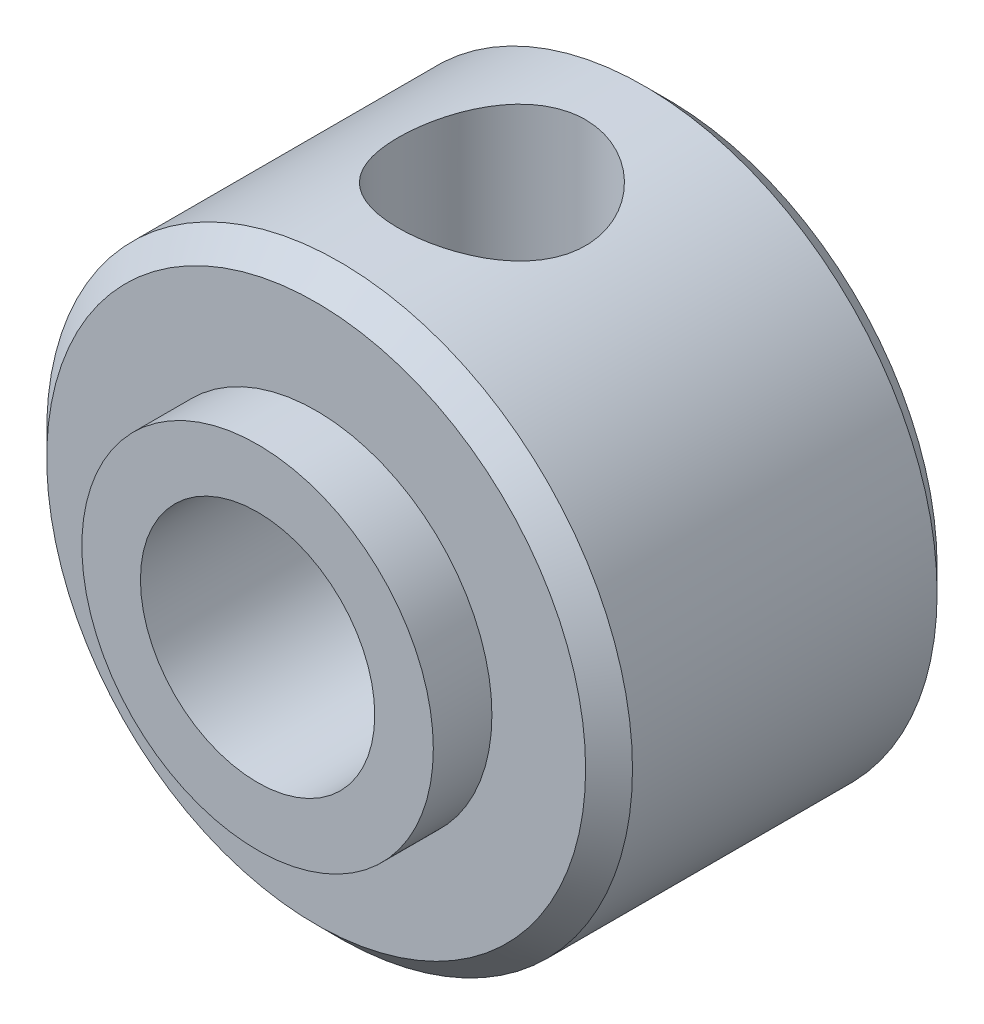
from build123d import *

# Parameters (mm, degrees)
SKETCH1_R           = 2.5
SKETCH1_R_2         = 1
BOSS_EXTRUDE1_DEPTH = 1.5
SKETCH2_R           = 1.5
SKETCH2_R_2         = 1
BOSS_EXTRUDE2_DEPTH = 0.5
SKETCH3_W           = 0.8
SKETCH3_H           = 2.5
CHAMFER1_SIZE       = 0.2


with BuildPart() as part:
    # Sketch1 → Boss-Extrude1 (new, symmetric)
    with BuildSketch(Plane.XY):
        Circle(SKETCH1_R)
        Circle(SKETCH1_R_2, mode=Mode.SUBTRACT)
    extrude(amount=BOSS_EXTRUDE1_DEPTH, both=True)

    # Sketch2 → Boss-Extrude2 (add)
    with BuildSketch(Plane.XY.offset(1.5)):
        Circle(SKETCH2_R)
        Circle(SKETCH2_R_2, mode=Mode.SUBTRACT)
    extrude(amount=BOSS_EXTRUDE2_DEPTH)

    # Sketch3 → M2 Tapped Hole1 (revolve, cut)
    with BuildSketch(Plane(origin=(0, 0, 0), x_dir=(0, 0, -1), z_dir=(1, 0, 0))):
        with Locations((0.4, 1.25)):
            Rectangle(SKETCH3_W, SKETCH3_H)
    revolve(axis=Axis((0, -6.35, 0), (0, 1, 0)), mode=Mode.SUBTRACT)

    # Chamfer1
    chamfer1_edges = [part.edges().sort_by_distance(p)[0] for p in [
        (-2.5, 0, -1.5),
        (-2.5, 0, 1.5),
    ]]
    chamfer(chamfer1_edges, length=CHAMFER1_SIZE)


solid = part.part
